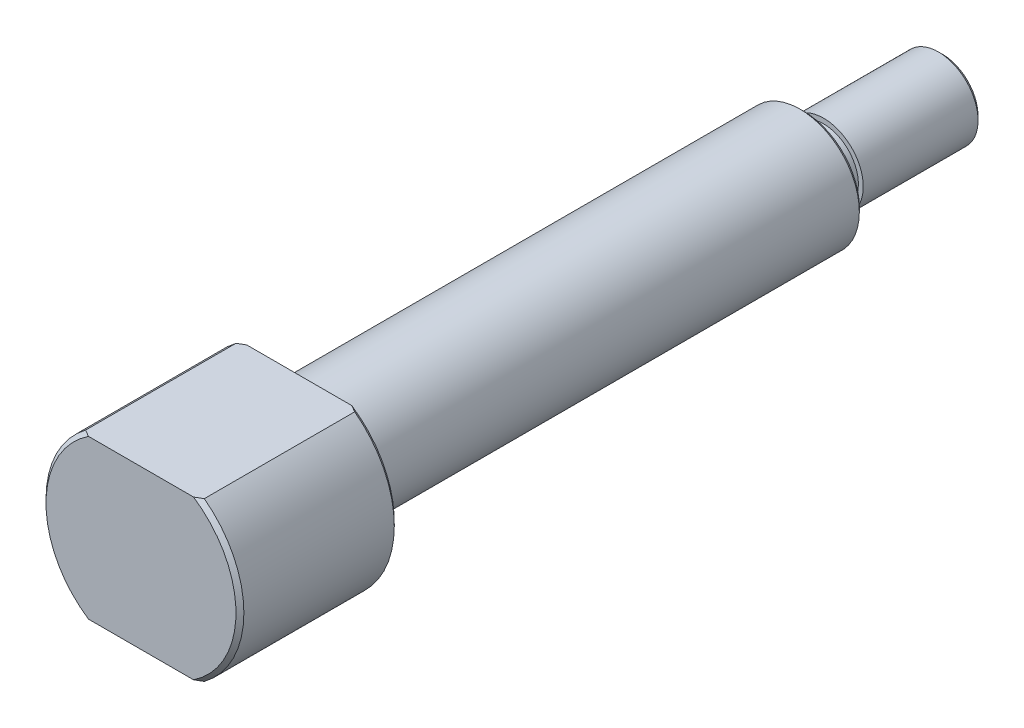
from build123d import *

# Parameters (mm, degrees)
SKETCH_1_R          = 3
EXTRUDE_1_DEPTH     = 12.75
CHAMFER_1_SIZE      = 0.2
SKETCH_2_R          = 2
EXTRUDE_2_DEPTH     = 7
CHAMFER_2_SIZE      = 0.2
SKETCH_3_R          = 5
EXTRUDE_3_DEPTH     = 8
CHAMFER_3_SIZE      = 0.2
CUT_EXTRUDE_1_REACH = 43.113
SKETCH_4_W          = 22.304994934
SKETCH_4_H          = 6.13630865
SKETCH_4_W_2        = 24.691337186
SKETCH_4_H_2        = 5.746701752
SKETCH_5_OUTSIDE_W  = 20.496
SKETCH_5_OUTSIDE_H  = 18.496
SKETCH_5_OUTSIDE_R  = 1.75
CUT_EXTRUDE_2_DEPTH = 1


with BuildPart() as part:
    # 草图1 → 凸台-拉伸1 (new, symmetric)
    with BuildSketch(Plane.XY):
        Circle(SKETCH_1_R)
    extrude(amount=EXTRUDE_1_DEPTH, both=True)

    # 倒角1
    chamfer_1_edges = [part.edges().sort_by_distance(p)[0] for p in [
        (-3, 0, -12.75),
    ]]
    chamfer(chamfer_1_edges, length=CHAMFER_1_SIZE)

    # 草图2 → 凸台-拉伸2 (add)
    with BuildSketch(Plane(origin=(0, 0, -12.75), x_dir=(-1, 0, 0), z_dir=(0, 0, -1))):
        with Locations(Location((0, 0, 0), (0, 0, 180))):
            Circle(SKETCH_2_R)
    extrude(amount=EXTRUDE_2_DEPTH)

    # 倒角2
    chamfer_2_edges = [part.edges().sort_by_distance(p)[0] for p in [
        (-2, 0, -19.75),
    ]]
    chamfer(chamfer_2_edges, length=CHAMFER_2_SIZE)

    # 草图3 → 凸台-拉伸3 (add)
    with BuildSketch(Plane.XY.offset(12.75)):
        Circle(SKETCH_3_R)
    extrude(amount=EXTRUDE_3_DEPTH)

    # 倒角3
    chamfer_3_edges = [part.edges().sort_by_distance(p)[0] for p in [
        (-5, 0, 12.75),
        (-5, 0, 20.75),
    ]]
    chamfer(chamfer_3_edges, length=CHAMFER_3_SIZE)

    # 切除-拉伸1: up to this face of the body (flat: up to its plane)
    cut_extrude_1_end = Plane(part.part.faces().sort_by_distance((-4.664235498, 0, 12.75))[0])
    # 草图4 → 切除-拉伸1 (cut, up to the picked face)
    with BuildSketch(Plane.XY.offset(20.75), mode=Mode.PRIVATE) as cut_extrude_1_sk1:
        with Locations((-4.583903449, 7.068154325)):
            Rectangle(SKETCH_4_W, SKETCH_4_H)
    cut_extrude_1_tool1 = split(extrude(cut_extrude_1_sk1.sketch, amount=-CUT_EXTRUDE_1_REACH, mode=Mode.PRIVATE), bisect_by=cut_extrude_1_end, keep=Keep.BOTH, mode=Mode.PRIVATE)
    # 草图4 → 切除-拉伸1 (cut, up to the picked face)
    with BuildSketch(Plane.XY.offset(20.75), mode=Mode.PRIVATE) as cut_extrude_1_sk2:
        with Locations((6.130286257, -6.873350876)):
            Rectangle(SKETCH_4_W_2, SKETCH_4_H_2)
    cut_extrude_1_tool2 = split(extrude(cut_extrude_1_sk2.sketch, amount=-CUT_EXTRUDE_1_REACH, mode=Mode.PRIVATE), bisect_by=cut_extrude_1_end, keep=Keep.BOTH, mode=Mode.PRIVATE)
    add(cut_extrude_1_tool1.solids().sort_by(Axis((-4.583903, 7.068154, 20.75), (0, 0, -1)))[0], mode=Mode.SUBTRACT)
    add(cut_extrude_1_tool2.solids().sort_by(Axis((6.130286, -6.873351, 20.75), (0, 0, -1)))[0], mode=Mode.SUBTRACT)

    # 草图5 outside → 切除-拉伸2 (cut)
    with BuildSketch(Plane(origin=(0, 0, -12.75), x_dir=(-1, 0, 0), z_dir=(0, 0, -1))):
        Rectangle(SKETCH_5_OUTSIDE_W, SKETCH_5_OUTSIDE_H)
        Circle(SKETCH_5_OUTSIDE_R, mode=Mode.SUBTRACT)
    extrude(amount=CUT_EXTRUDE_2_DEPTH, mode=Mode.SUBTRACT)


solid = part.part
